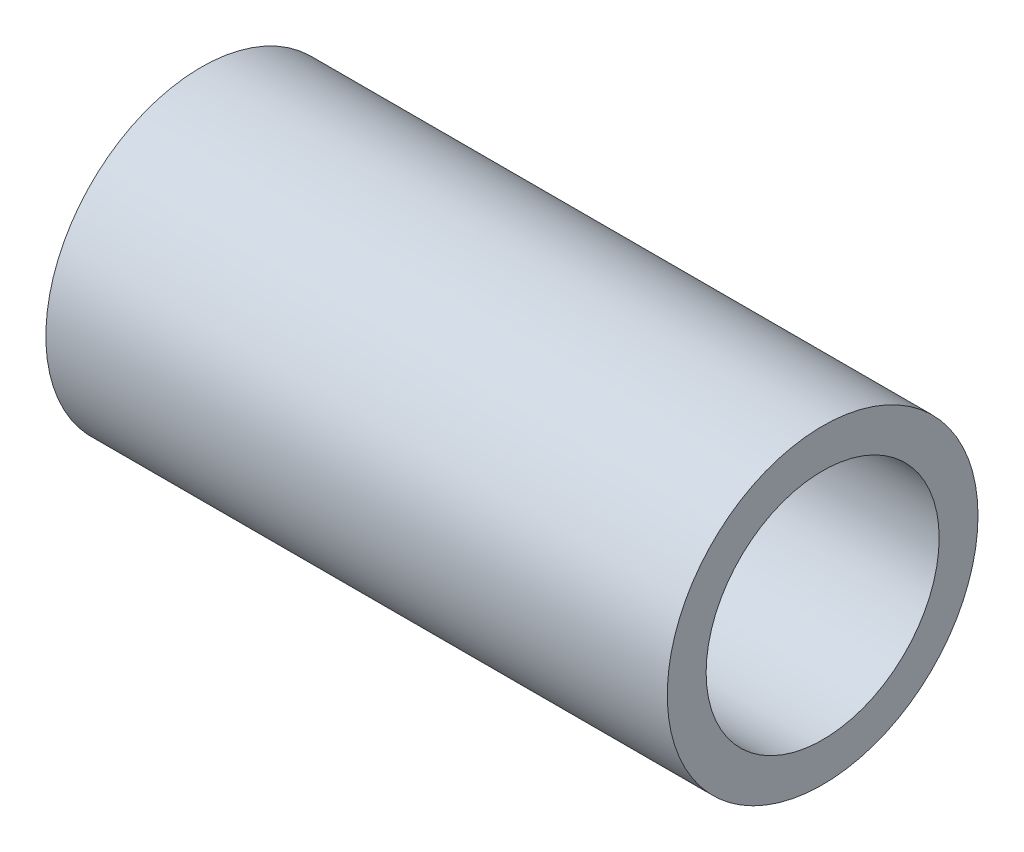
SolidWorks part; units mm, degrees
ref_plane "Front Plane" through (0, 0, 0) normal (0, 0, 1) x (1, 0, 0)
ref_plane "Top Plane" through (0, 0, 0) normal (0, 1, 0) x (1, 0, 0)
ref_plane "Right Plane" through (0, 0, 0) normal (1, 0, 0) x (0, 0, -1)
other "Configuration Table"
sketch "Sketch1" plane through (0, 0, 0) normal (1, 0, 0) x (0, 0, -1)
  circle A0 centre (0, 0) radius 30
  circle A1 centre (0, 0) radius 40
  dimension "D1" = 80
  dimension "D2" = 60
extrude "Boss-Extrude1" add sketch "Sketch1" along normal blind 160
